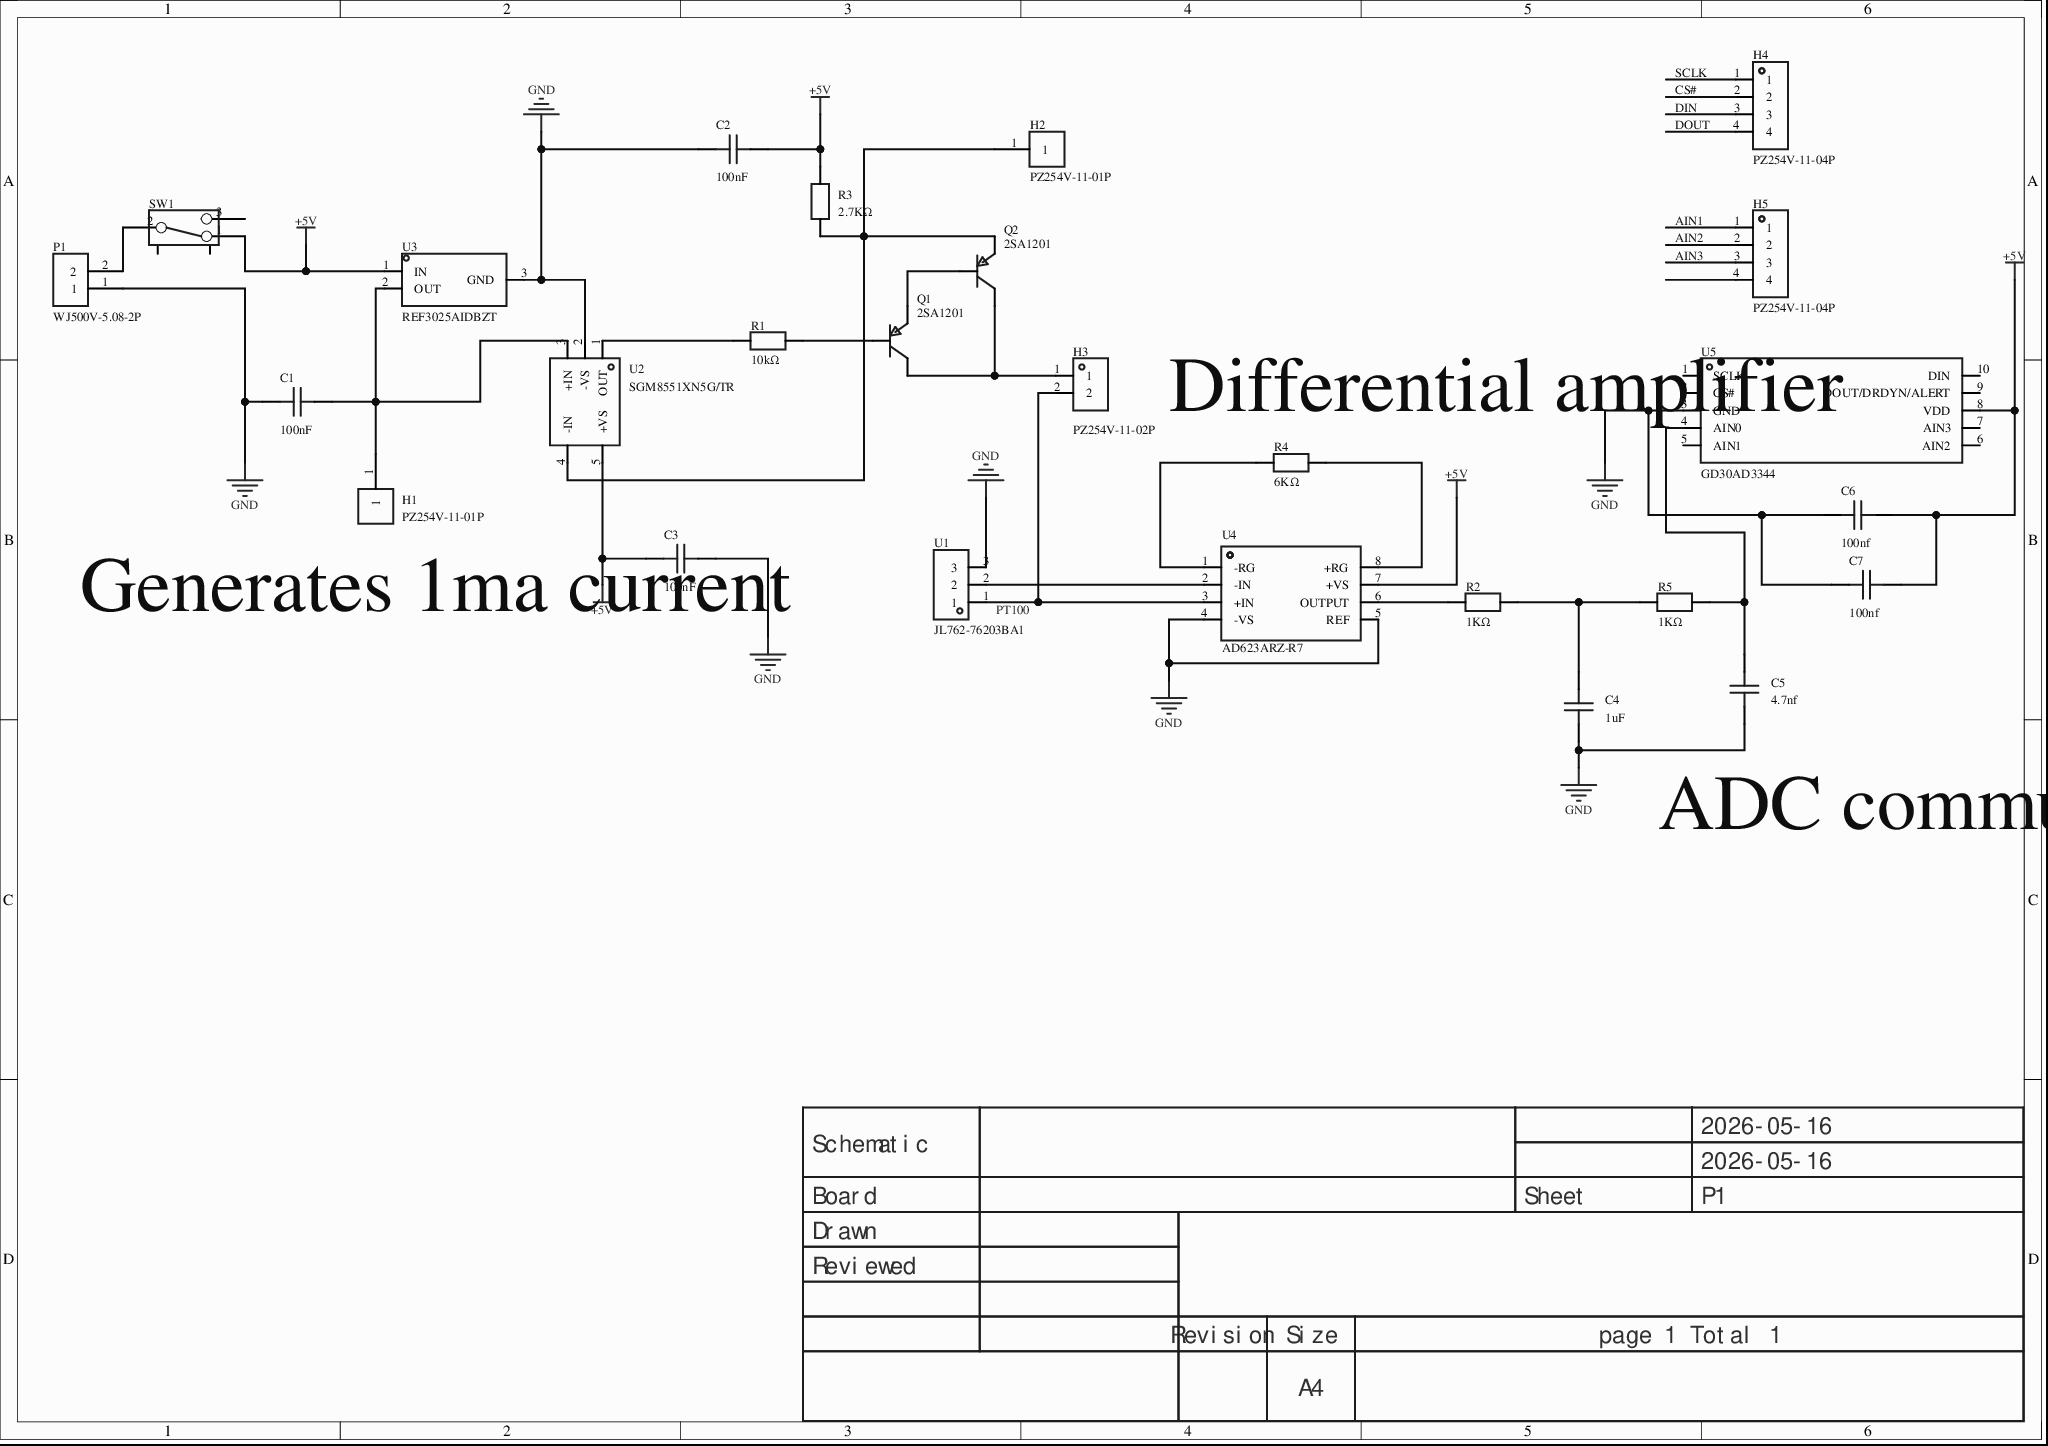
[diagram p0: MISC52115-3.schdoc]
# Altium project MISC52115-2.PrjPcb
1 sheet, 26 parts. Net scope: global (net labels, ports and power ports of the same name join across sheets).
Board file: MISC52115.pcbdoc

## Sheet MISC52115-3.schdoc
size 297 x 209 mm; Version: V1.0; @Project Name: MISC52115; @Update Date: 2026-05-16; @Create Date: 2026-05-16; @Board Name: MISC52115; @Create Time: 20:58:32; @Page Count: 1; @Page No: 1; @Schematic Name: MISC52115; @Update Time: 20:58:32; Size: A4

### Parts
C1  100nF  [CAP-SMD_L2.0-W1.25]
C2  100nF  [CAP-SMD_L2.0-W1.25]
C3  100nF  [CAP-SMD_L2.0-W1.25]
C4  1uF  [CAP-SMD_L2.0-W1.25]
C5  4.7nf  [CAP-SMD_L2.0-W1.25]
C6  100nf  [CAP-SMD_L2.0-W1.25]
C7  100nf  [CAP-SMD_L2.0-W1.25]
H1  PZ254V-11-01P  [HDR-TH_1P-P2.54-V-M]
H2  PZ254V-11-01P  [HDR-TH_1P-P2.54-V-M]
H3  PZ254V-11-02P  [HDR-TH_2P-P2.54-V-M]
H4  PZ254V-11-04P  [HDR-TH_4P-P2.54-V-M]
H5  PZ254V-11-04P  [HDR-TH_4P-P2.54-V-M]
P1  WJ500V-5.08-2P  [CONN-TH_2P-P5.00_WJ500V-5.08-2P]
Q1  2SA1201  [SOT-89-3_L4.5-W2.5-P1.50-LS4.2-BR]
Q2  2SA1201  [SOT-89-3_L4.5-W2.5-P1.50-LS4.2-BR]
R1  10kΩ  [R0805]
R2  1KΩ  [R1206]
R3  2.7KΩ  [R1206]
R4  6KΩ  [R1206]
R5  1KΩ  [R1206]
SW1  (no value)  [拨动开关]
U1  JL762-76203BA1  [CONN-TH_JL762-76203BA1]
U2  SGM8551XN5G/TR  [SOT-23-5_L3.0-W1.7-P0.95-LS2.8-BL]
U3  REF3025AIDBZT  [SOT-23-3_L3.0-W1.7-P0.95-LS2.9-BR]
U4  AD623ARZ-R7  [SOIC-8_L5.0-W4.0-P1.27-LS6.0-BL]
U5  GD30AD3344  [MSOP-10_L3.0-W3.0-P0.50-LS5.0-BL]

### Nets
+5V: C2.2 C3.1 C6.1 C7.1 R3.2 SW1.1 U2.5(+VS) U3.1(IN) U4.7(+VS) U5.8(VDD)
GND: C1.1 C2.1 C3.2 C4.1 C5.1 C6.2 C7.2 P1.1 U1.3 U2.2(-VS) U3.3(GND) U4.4(-VS) U4.5(REF) U5.3(GND)
PT100: H3.2 U1.1 U4.3(+IN)
NetC1_2: C1.2 H1.1 U2.3(+IN) U3.2(OUT)
NetC4_2: C4.2 R2.2 R5.1
NetC5_2: C5.2 R5.2 U5.4(AIN0)
NetH2_1: H2.1 Q2.3(E) R3.1 U2.4(-IN)
NetH3_1: H3.1 Q1.2(C) Q2.2(C)
NetP1_2: P1.2 SW1.2
NetQ1_1: Q1.1(B) R1.2
NetQ1_3: Q1.3(E) Q2.1(B)
NetR1_1: R1.1 U2.1(OUT)
NetR2_1: R2.1 U4.6(OUTPUT)
NetR4_1: R4.1 U4.8(+RG)
NetR4_2: R4.2 U4.1(-RG)
NetU1_2: U1.2 U4.2(-IN)

Not connected (* = marked no-connect by the designer): H4 1 2 3 4; H5 1 2 3 4; SW1 3 4 5; U5 1(SCLK) 2(CS#) 5(AIN1) 6(AIN2) 7(AIN3) 9(DOUT/DRDYN/ALERT) 10(DIN)

### Notes on the sheet
- (near H4) SCLK
- (near H4) CS#
- (near H4) DIN
- (near H4) DOUT
- (near H5) AIN1
- (near H5) AIN2
- (near H5) AIN3
- (near U5) Differential amplifier
- (near C3) Generates 1ma current
- (near C5) ADC communication
- 2026-05-16
- Schematic
- Board
- Sheet
- P1
- Drawn
- Reviewed
- Revision
- Size
- A4
- page 1 Total 1

### Library data of the parts
C1-C3 = FCC0805B104K500DT: Capacitance:100nF;Tolerance:±10%;Rated voltage:50V;Temperature coefficient:X7R;; Manufacturer: FOJAN(富捷); AddInBom: yes; ModelId: dce19e309e9b4209af79576cb8c62f2f0819f05c4eef4c71ace90d822a990e87; ModelName: CAP-SMD_L2.0-W1.3-H1.3; ModelTransform: 78.74,49.2125,0,0,0,0,0,0,0; Tolerance: ±10%; Voltage Rating: 50V; Temperature Coefficient: X7R; Symbol: FCC0805B104K500DT; Device: FCC0805B104K500DT; LCSC Part Name: 100nF ±10% 50V; SupplierPart: C5137467; ManufacturerPart: FCC0805B104K500DT; Supplier Footprint: 0805; JLCPCB Part Class: Extended Part; Datasheet: https://item.szlcsc.com/datasheet/FCC0805B104K500DT/5746969.html; Supplier: LCSC; ConvertToPcb: yes; FootprintName: CAP-SMD_L2.0-W1.25; Value: 100nF
C4-C7 = FCC0805B104K500DT: Capacitance:100nF;Tolerance:±10%;Rated voltage:50V;Temperature coefficient:X7R;; Manufacturer: FOJAN(富捷); 3D Model: dce19e309e9b4209af79576cb8c62f2f0819f05c4eef4c71ace90d822a990e87; 3D Model Transform: 78.74,49.2125,0,0,0,0,0,0,0; Tolerance: ±10%; Voltage Rating: 50V; Temperature Coefficient: X7R; AddInBom: yes; ModelName: CAP-SMD_L2.0-W1.3-H1.3; Symbol: FCC0805B104K500DT; Device: FCC0805B104K500DT; LCSC Part Name: 100nF ±10% 50V; Manufacturer Part: FCC0805B104K500DT; Supplier Footprint: 0805; JLCPCB Part Class: Extended Part; Datasheet: https://item.szlcsc.com/datasheet/FCC0805B104K500DT/5746969.html; Supplier: LCSC; ConvertToPcb: yes; FootprintName: CAP-SMD_L2.0-W1.25
  C4: Value: 1uF
  C5: Value: 4.7nf
  C6 C7: Value: 100nf
H1 H2 = PZ254V-11-01P: Pin structure:1x1P;Pitch:2.54mm;Row spacing:-;Round/square pin:Square pin;Mounting style:Through-hole;Rows:Single row;Total pin count:1P;Rated current:3A;Rated voltage:250V;Mating length:6mm;Housing height:2.5mm;Tail length:3mm;Contact material:Brass;Contact plating:-;Operating temperature:-40℃~+105℃;Color:Black;; Manufacturer: XFCN(兴飞); AddInBom: yes; ModelId: efa57846279b44bfa0a28253a2c74e330819f05c4eef4c71ace90d822a990e87; ModelName: HDR2.54-M-LI-1X1P; ModelTransform: 100,100,0,0,0,0,0,0,-118.11; Pin Structure: 1x1P; Pitch: 2.54mm; Current Rating: 3A; Voltage Rating (Max): 250V; Symbol: PZ254V-11-01P; Device: PZ254V-11-01P; LCSC Part Name: 1x1P 间距:2.54mm 方针 直插; SupplierPart: C492400; ManufacturerPart: PZ254V-11-01P; Supplier Footprint: 插件,P=2.54mm; JLCPCB Part Class: Extended Part; Datasheet: https://item.szlcsc.com/datasheet/PZ254V-11-01P/502956.html; Supplier: LCSC; ConvertToPcb: yes; FootprintName: HDR-TH_1P-P2.54-V-M; Row Spacing: -; Circluar Pins/Square Pins: Square pin; Mounting Type: Through-hole; Number of Rows: Single row; Number of Pins: 1P; Length of Mating Pin: 6mm; Insulation Height: 2.5mm; Length of End Connection Pin: 3mm; Contact Material: Brass; Contact Plating: -; Operating Temperature: -40℃~+105℃; Color: Black
H3 = PZ254V-11-02P: Pin structure:1x2P;Pitch:2.54mm;Row spacing:-;Round/square pin:Square pin;Mounting style:Through-hole;Rows:Single row;Total pin count:2P;Rated current:3A;Rated voltage:250V;Mating length:6mm;Housing height:2.5mm;Tail length:3mm;Contact material:Brass;Contact plating:-;Operating temperature:-40℃~+105℃;Color:Black;; Manufacturer: XFCN(兴飞); AddInBom: yes; ModelId: e35305ec3aa84b66b849f914b715e73f0819f05c4eef4c71ace90d822a990e87; ModelName: HDR2.54-M-LI-1X2P; ModelTransform: 200,100,0,0,0,0,0,0,-118.11; Pin Structure: 1x2P; Pitch: 2.54mm; Current Rating: 3A; Voltage Rating (Max): 250V; Symbol: PZ254V-11-02P; Device: PZ254V-11-02P; LCSC Part Name: 1x2P 间距:2.54mm 方针 直插; SupplierPart: C492401; ManufacturerPart: PZ254V-11-02P; Supplier Footprint: 插件,P=2.54mm; JLCPCB Part Class: Extended Part; Datasheet: https://item.szlcsc.com/datasheet/PZ254V-11-02P/502957.html; Supplier: LCSC; ConvertToPcb: yes; FootprintName: HDR-TH_2P-P2.54-V-M; Row Spacing: -; Circluar Pins/Square Pins: Square pin; Mounting Type: Through-hole; Number of Rows: Single row; Number of Pins: 2P; Length of Mating Pin: 6mm; Insulation Height: 2.5mm; Length of End Connection Pin: 3mm; Contact Material: Brass; Contact Plating: -; Operating Temperature: -40℃~+105℃; Color: Black
H4 H5 = PZ254V-11-04P: Pin structure:1x4P;Pitch:2.54mm;Row spacing:-;Round/square pin:Square pin;Mounting style:Through-hole;Rows:Single row;Total pin count:4P;Rated current:3A;Rated voltage:250V;Mating length:6mm;Housing height:2.5mm;Tail length:3mm;Contact material:-;Operating temperature:-40℃~+105℃;Color:Black;; Manufacturer: XFCN(兴飞); Symbol: PZ254V-11-04P_C2691448; AddInBom: yes; ModelId: 112f4d05e8d64e99ab9a333894bea4f90819f05c4eef4c71ace90d822a990e87; ModelName: HDR-TH_4P-P2.54-M-LI-1X4P; ModelTransform: 399.999,104.7242,0,0,0,0,0,0,-118.11; Pin Structure: 1x4P; Pitch: 2.54mm; Current Rating: 3A; Voltage Rating (Max): 250V; Device: PZ254V-11-04P; LCSC Part Name: 1x4P 间距:2.54mm 方针 直插; SupplierPart: C2691448; ManufacturerPart: PZ254V-11-04P; Supplier Footprint: 插件,P=2.54mm; JLCPCB Part Class: Extended Part; Datasheet: https://item.szlcsc.com/datasheet/PZ254V-11-04P/2801085.html; Supplier: LCSC; ConvertToPcb: yes; FootprintName: HDR-TH_4P-P2.54-V-M; Row Spacing: -; Circluar Pins/Square Pins: Square pin; Mounting Type: Through-hole; Number of Rows: Single row; Number of Pins: 4P; Length of Mating Pin: 6mm; Insulation Height: 2.5mm; Length of End Connection Pin: 3mm; Contact Material: -; Operating Temperature: -40℃~+105℃; Color: Black
P1 = WJ500V-5.08-2P: Structure:1x2P;Pitch:5.08mm;Color:Green;Mounting style:Through-hole;Rated current:18A;Rated voltage:250V;Rows:1;Wire gauge - AWG:14~30;Wire gauge - mm2:2.5;Pins per row:2;Contact material:-;Contact plating:-;Operating temperature range:-40℃~+105℃;Soldering temperature (max):-;; Manufacturer: KANGNEX(康奈克斯电气); Symbol: WJ500V-5.08-2P-14-00A; AddInBom: yes; ModelId: 0f4a503c8d3b4ae19ed61267f5e9a1d70819f05c4eef4c71ace90d822a990e87; ModelTransform: 423.621,393.7,0,0,0,0,-11.811,19.685,-137.795; Structure: 1x2P; Pitch: 5.08mm; Current Rating (Max): 18A; Voltage Rating (Max): 250V; Wire Gauge - AWG: 14~30; Wire Gauge - mm2: 2.5; Number of PINs Per Row: 2; Screw Specification: M2.5; Device: WJ500V-5.08-2P; LCSC Part Name: 1x2P 5.08mm 直插 排数:1 每排P数:2; SupplierPart: C8465; ManufacturerPart: WJ500V-5.08-2P; Supplier Footprint: 插件,P=5.08mm; JLCPCB Part Class: Extended Part; Datasheet: https://atta.szlcsc.com/upload/public/pdf/source/20191225/C8465_02D34CE5B5B4A53DF5891601D97FA9F4.pdf; Supplier: LCSC; ConvertToPcb: yes; FootprintName: CONN-TH_2P-P5.00_WJ500V-5.08-2P; ModelName: CONN-TH_2P-P5.00_WJ500V-5.08-2P; Color: Green; Mounting Style: Through-hole; Number of Pins: 2P; Number of Rows: 1; Contact Material: -; Contact Plating: -; Operating Temperature Range: -40℃~+105℃; Soldering Temperature(Max): -
Q1 Q2 = 2SA1201: Transistor type:PNP;Collector current (Ic):800mA;Collector-emitter breakdown voltage (Vceo):120V;Power dissipation (Pd):500mW;DC current gain (hFE):240@100mA,5V;; Manufacturer: R+O(宏嘉诚); Symbol: 2SA1201_C41375121; AddInBom: yes; ModelId: 6db690b7897d4d18a30d90c1b89525ee0819f05c4eef4c71ace90d822a990e87; ModelName: SOT-89-3_L4.3-W2.5-H1.6-LS4.1-P1.50; ModelTransform: 161.417,169.291,0,180,0,0,-11.808,0,0; type: PNP; Current - Collector(Ic): 800mA; Collector - Emitter Voltage VCEO: 120V; Pd - Power Dissipation: 500mW; Transition frequency(fT): 120MHz; Current - Collector Cutoff: 100nA; Vce Saturation(VCE(sat)): 1V@500mA,50mA; Device: 2SA1201; LCSC Part Name: PNP 电流:800mA 电压:120V; SupplierPart: C41375121; ManufacturerPart: 2SA1201; Supplier Footprint: SOT-89; JLCPCB Part Class: Extended Part; Datasheet: https://item.szlcsc.com/datasheet/2SA1201/43142121.html; Supplier: LCSC; ConvertToPcb: yes; FootprintName: SOT-89-3_L4.5-W2.5-P1.50-LS4.2-BR; DC Current Gain: 240@100mA,5V; Operating Temperature: -; Emitter-Base Voltage(Vebo): 5V
R1 = FRC0805J103TS: Resistor type:Thick film resistor;Resistance:10kΩ;Tolerance:±5%;Power:125mW;Working voltage:150V;Temperature coefficient:±100ppm/℃;; Manufacturer: FOJAN(富捷); AddInBom: yes; ModelId: 37a81e68749a4138bd2dfa6897b24b850819f05c4eef4c71ace90d822a990e87; ModelName: R0805_L2.0-W1.3-H0.6; ModelTransform: 78.74,51.181,0,0,0,0,0,-0.0005,0; Tolerance: ±5%; Power(Watts): 125mW; Voltage-Supply(Max): 150V; Symbol: FRC0805J103TS; Device: FRC0805J103TS; LCSC Part Name: 10kΩ ±5% 125mW 厚膜电阻; SupplierPart: C2930231; ManufacturerPart: FRC0805J103TS; Supplier Footprint: 0805; JLCPCB Part Class: Extended Part; Supplier: LCSC; ConvertToPcb: yes; FootprintName: R0805; Type: Thick film resistor; Value: 10kΩ; Temperature Coefficient: ±100ppm/℃; Operating Temperature: -55℃~+155℃
R2 R4 R5 = HoJLRH1206-1W-500mR-1%: Resistor type:Thin film resistor;Resistance:500mΩ;Tolerance:±1%;Power:1W;Temperature coefficient:±100ppm/℃;; Manufacturer: Milliohm(毫欧); 3D Model: 89a1f13db2384da588040e0b3c55bf660819f05c4eef4c71ace90d822a990e87; 3D Model Transform: 125.984,62.992,0,0,0,0,0,0,0; Tolerance: ±1%; Power(Watts): 1W; AddInBom: yes; ModelName: R1206_L3.2-W1.6-H0.6; Symbol: HOJLRH1206-1W-500MR-1%; Device: HoJLRH1206-1W-500mR-1%; LCSC Part Name: 薄膜电阻 500mΩ ±1% 1W; Manufacturer Part: HoJLRH1206-1W-500mR-1%; Supplier Footprint: 1206; Datasheet: https://item.szlcsc.com/datasheet/HoJLRH1206-1W-500mR-1%2525/48731416.html; Supplier: LCSC; Type: Thin film resistor; Temperature Coefficient: ±100ppm/℃; Operating Temperature: -55℃~+155℃; ConvertToPcb: yes; FootprintName: R1206
  R2 R5: Value: 1KΩ
  R4: Value: 6KΩ
R3 = HoJLRH1206-1W-500mR-1%: Resistor type:Thin film resistor;Resistance:500mΩ;Tolerance:±1%;Power:1W;Temperature coefficient:±100ppm/℃;; Manufacturer: Milliohm(毫欧); AddInBom: yes; ModelId: 89a1f13db2384da588040e0b3c55bf660819f05c4eef4c71ace90d822a990e87; ModelName: R1206_L3.2-W1.6-H0.6; ModelTransform: 125.984,62.992,0,0,0,0,0,0,0; Tolerance: ±1%; Power(Watts): 1W; Symbol: HOJLRH1206-1W-500MR-1%; Device: HoJLRH1206-1W-500mR-1%; Value: 2.7KΩ; LCSC Part Name: 薄膜电阻 500mΩ ±1% 1W; ManufacturerPart: HoJLRH1206-1W-500mR-1%; Supplier Footprint: 1206; Datasheet: https://item.szlcsc.com/datasheet/HoJLRH1206-1W-500mR-1%2525/48731416.html; Supplier: LCSC; ConvertToPcb: yes; FootprintName: R1206; Type: Thin film resistor; Temperature Coefficient: ±100ppm/℃; Operating Temperature: -55℃~+155℃
SW1 = 拨动开关_正: Symbol: Toggle switch; Device: Toggle switch_positive; ConvertToPcb: yes; ModelId: 4321fe59a4074cbfb4989553f297c68f0819f05c4eef4c71ace90d822a990e87; ModelName: SW-TH_SS-12D02-VG4; ModelTransform: 370.09,208.7,472.35,0,0,0,0,0,-110; AddInBom: yes; Supplier Footprint: 插件; FootprintName: Toggle switch
U1 = JL762-76203BA1: Barrier type:Three-sided;Pitch:7.62mm;Structure:1x3P;Mounting style:Through-hole;Pin location:Edge pin;Rows:1;Pins per row:3;Rated current:20A;Rated voltage:300V;Wire gauge - AWG:14~22;Wire gauge - mm2:-;Operating temperature:-40℃~+105℃;Color:Black;; Manufacturer: JILN(锦凌); AddInBom: yes; ModelId: 7ff898602bbe4f56ba0b8fd68832b6590819f05c4eef4c71ace90d822a990e87; ModelTransform: 947.242,602.361,0,0,0,0,0,-123.622,-149.606; Pitch: 7.62mm; Number of Positions or Pins: 1x3P; Number of PINs Per Row: 3; Screw Specification: M3.5; Current Rating: 20A; Voltage Rating (Max): 300V; Wire Gauge - AWG: 14~22; Symbol: JL762-76203BA1; Device: JL762-76203BA1; LCSC Part Name: 7.62mm 1x3P 直插 边脚 排数:1 每排P数:3; SupplierPart: C424382; ManufacturerPart: JL762-76203BA1; Supplier Footprint: 插件,P=7.62mm; JLCPCB Part Class: Extended Part; Datasheet: https://item.szlcsc.com/datasheet/JL762-76203BA1/417447.html; Supplier: LCSC; ConvertToPcb: yes; FootprintName: CONN-TH_JL762-76203BA1; ModelName: CONN-TH_JL762-76203BA1; Barrier Type: Three-sided; Mounting Type: Through-hole; Pin Location: Edge pin; Number of Pins: 3P; Number of Rows: 1; Wire Gauge - mm2: -; Operating Temperature: -40℃~+105℃; Color: Black
U2 = SGM8551XN5G/TR: Amplifier count:-;; Manufacturer: SGMICRO(圣邦微); AddInBom: yes; ModelId: 0a2a1b8f50944f73965918ad6e5fe1670819f05c4eef4c71ace90d822a990e87; ModelName: SOT-23-5_L2.9-W1.6-H1.1-LS2.8-P0.95; ModelTransform: 118.60433,114.173,0,90,0,0,0.0005,0.0005,0; Symbol: SGM8551XN5G/TR; Device: SGM8551XN5G/TR; LCSC Part Name: SGM8551XN5G/TR; SupplierPart: C83748; ManufacturerPart: SGM8551XN5G/TR; Supplier Footprint: SOT-23-5; JLCPCB Part Class: Extended Part; Datasheet: https://atta.szlcsc.com/upload/public/pdf/source/20241203/4E0FBB26B357572199B7BC85CD4D9122.pdf; Supplier: LCSC; ConvertToPcb: yes; FootprintName: SOT-23-5_L3.0-W1.7-P0.95-LS2.8-BL; Number of Channels: -
U3 = REF3025AIDBZT: Output type:Fixed;Operating voltage:2.55V~5.5V;Output voltage:2.5V;Output current:25mA;Accuracy:±0.2%;; Manufacturer: TI(德州仪器); AddInBom: yes; ModelId: 89cb27a44ab2466697082bb9fd73a7d00819f05c4eef4c71ace90d822a990e87; ModelName: SOT-23-3L_L2.9-W1.6-H1.1-LS2.8-P0.95; ModelTransform: 114.173,110.236,0,90,0,0,0,0,0; Output Type: Fixed; Output Voltage: 2.5V; Output Current: 25mA; Tolerance: ±0.2%; Temperature Coefficient: 75ppm/℃; Reference Type: Series; Quiescent Current: 42uA; Noise - 1/10Hz to 10Hz: 28uVp-p; Noise - 10Hz to 10kHz: 80uVrms; Symbol: REF3025AIDBZT; Device: REF3025AIDBZT; LCSC Part Name: 2.55V~5.5V 串联 42uA 75ppm/℃; SupplierPart: C96625; ManufacturerPart: REF3025AIDBZT; Supplier Footprint: SOT-23; JLCPCB Part Class: Extended Part; Supplier: LCSC; ConvertToPcb: yes; FootprintName: SOT-23-3_L3.0-W1.7-P0.95-LS2.9-BR; Voltage - Supply: 2.55V~5.5V; Minimum Cathode Current for Regulation: -; Operating Temperature: -40℃~+125℃@(Ta)
U4 = AD623ARZ-R7: Amplifier count:Single;Common-mode rejection ratio (CMRR):80dB;Input bias current (Ib):25nA;Input offset voltage (Vos):200uV;Gain bandwidth product (GBP):-;Slew rate (SR):0.3V/us;Rail to rail:Rail-to-rail output;; Manufacturer: ADI(亚德诺); AddInBom: yes; ModelId: 7abc64c95a1a4a04a4ef38f9097c870b0819f05c4eef4c71ace90d822a990e87; ModelTransform: 192.913,236.22,0,0,0,0,0,0,0; Number of Channels: Single; Common Mode Rejection Ratio(CMRR): 80dB; Ib - Input Bias Current: 25nA; Vos - Input Offset Voltage: 200uV; Quiescent Current(Iq): 550uA; Symbol: AD623ARZ-R7; Device: AD623ARZ-R7; LCSC Part Name: 单电源、轨到轨、低成本仪表放大器; SupplierPart: C9676; ManufacturerPart: AD623ARZ-R7; Supplier Footprint: SOIC-8; JLCPCB Part Class: Extended Part; Datasheet: https://item.szlcsc.com/datasheet/AD623ARZ-R7/10206.html; Supplier: LCSC; ConvertToPcb: yes; FootprintName: SOIC-8_L5.0-W4.0-P1.27-LS6.0-BL; ModelName: SOIC-8_L5.0-W4.0-P1.27-LS6.0-BL; Gain Bandwidth Product: -; Slew Rate: 0.3V/us; Rail to Rail: Rail-to-rail output; Output Type: -; Operating Temperature: -40℃~+85℃
U5 = GD30AD3344: AddInBom: yes; ModelId: b42a31f9e1fa4643bc7ea573b9bba7ed0819f05c4eef4c71ace90d822a990e87; ModelName: MSOP-10_L3.0-W3.0-H1.1-LS5.0-P0.50; ModelTransform: 118.11,196.85,0,0,0,0,0,0,0; Symbol: GD30AD3344; Device: GD30AD3344; LCSC Part Name: GD30AD3344; SupplierPart: C9900209500; ManufacturerPart: GD30AD3344; Supplier Footprint: MSOP-10; Supplier: LCSC; ConvertToPcb: yes; FootprintName: MSOP-10_L3.0-W3.0-P0.50-LS5.0-BL